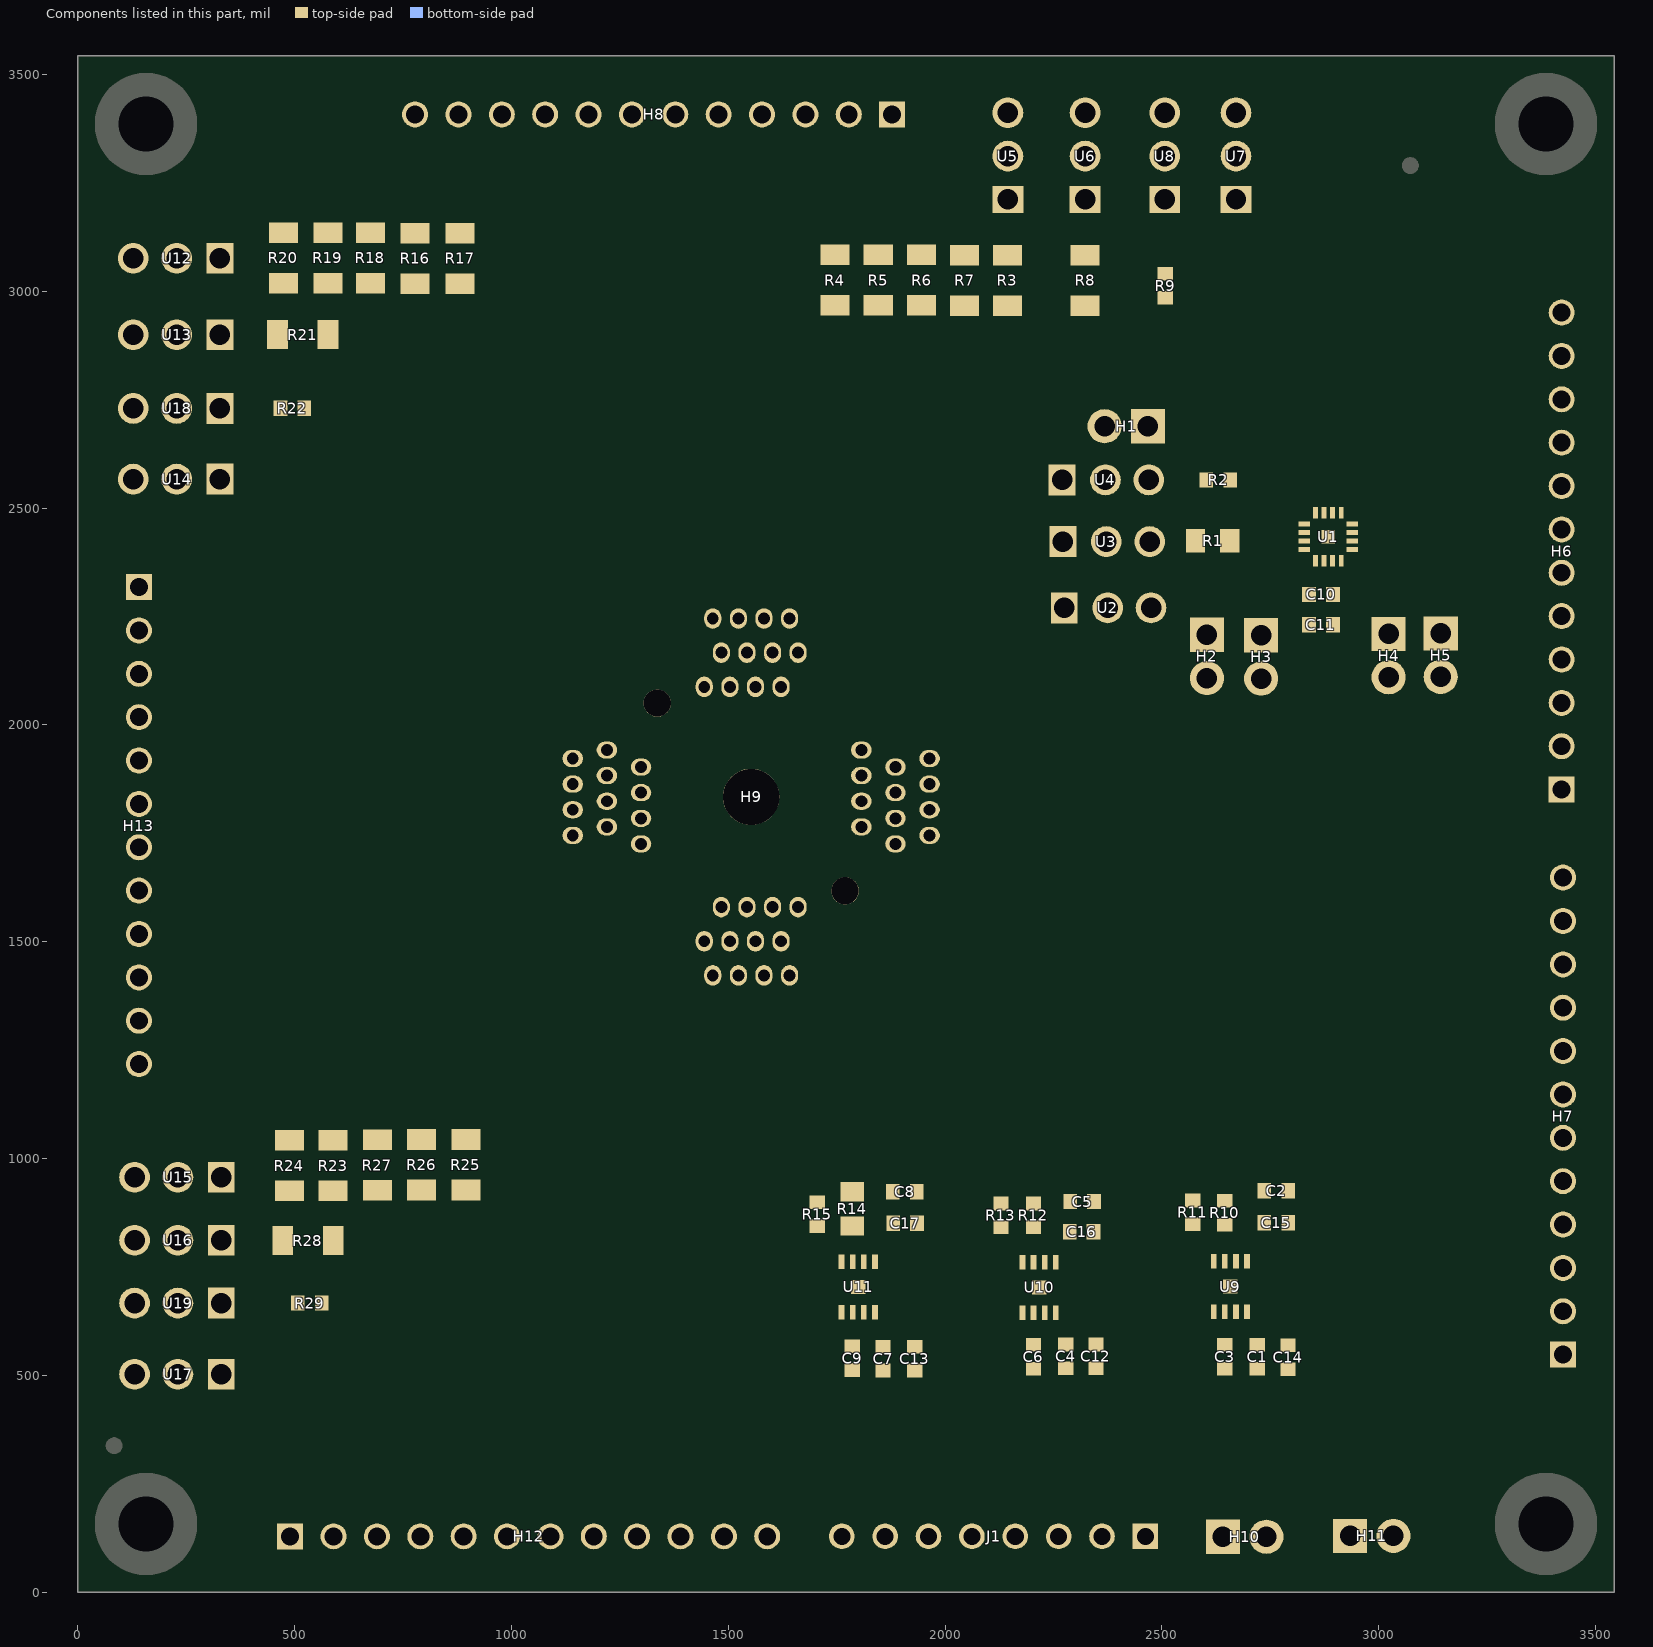
[diagram p0: the components of this part, seen from the top]
# Altium PCB MISC79022.pcbdoc (part 3 of 3)
Units mil, origin at the board's own origin, x right, y up, seen from the top; angles counter-clockwise.
Board outline 3543.31 x 3543.31 mil, 2 copper layers (Top Layer, Bottom Layer); 79 components, 75 nets, 320 pads, 1402 vias.

## Polygon pours and split planes (outlines as drawn)
AVSS on Top Layer "Bottom Layer-No Net" (solid, remove dead copper, pour order 1019): -259,3417.61 -237,3395.61 -237,-231.39 3714,-231.39 3804,-141.39 3860,-85.39 3860,70.61 3860,3854.61 3748,3966.61 3659,4055.61 3614,4055.61 -12,4055.61 -225,3842.61 -270,3797.61 -270,3551.61
3.3V on Top Layer "Bottom Layer-No Net" (solid, remove dead copper, pour order 1018): 2331,152 2331,81 2340,72 2351,61 2394,61 2797,61 2809,73 2818,82 2818,124 2818,276 2912,370 3013,471 3323,471 3444,471 3457,484 3464,491 3464,499 3464,576 3455,585 3437,585 3031,585 2967,649 2952,664 2696,664 2671,664 2668,661 2665,658 2665,652 2665,628 2670,623 2689,604 2689,585 2689,568 2696,561 2700,557 2719,557 2815,557 2833,539 2837,535 2837,521 2837,484 2815,462 2800,447 2686,447 2545,447 2515,477 2497,495 2497,546 2497,612 2468,641 2448,661 2256,661 2232,661 2229,658 2223,652 2223,646 2223,627 2237,613 2243,607 2243,595 2243,575 2255,563 2260,558 2269,558 2367,558 2379,546 2382,543 2382,528 2382,441 2354,413 2342,401 2293,401 2184,401 2143,442 2104,481 2104,545 2104,596 2075,625 2039,661 1841,661 1811,661 1808,658 1806,656 1806,652 1806,622 1818,610 1825,603 1825,594 1825,567 1833,559 1843,549 1852,549 1961,549 1976,534 1999,511 1999,477 1999,373 2020,352 2106,266 2181,266 2269,266 2308,227 2331,204 2331,153
LDO_AVDD on Top Layer "Bottom Layer-No Net" (solid, remove dead copper, pour order 1017): 2624,943 2624,894 2628,890 2634,884 2645,884 2675,884 2683,876 2690,869 2690,851 2690,825 2673,808 2664,799 2664,785 2664,751 2666,749 2668,747 2671,747 2726,747 2734,755 2754,775 2754,837 2754,988 2740,1002 2729,1013 2718,1013 2660,1013 2647,1000 2624,977 2624,944
LDO_DVDDIO on Top Layer "Bottom Layer-No Net" (solid, remove dead copper, pour order 1016): 2222,777 2222,750 2224,748 2227,745 2232,745 2281,745 2289,753 2306,770 2306,824 2306,968 2299,975 2293,981 2282,981 2199,981 2194,976 2183,965 2183,941 2183,894 2190,887 2195,882 2210,882 2225,882 2233,874 2240,867 2240,855 2240,817 2230,807 2222,799 2222,778
LDO_DVDD on Top Layer "Bottom Layer-No Net" (solid, remove dead copper, pour order 1015): 1806,781 1806,754 1808,752 1813,747 1818,747 1862,747 1866,751 1899,784 1899,845 1899,993 1882,1010 1875,1017 1860,1017 1760,1017 1755,1012 1748,1005 1748,975 1748,913 1760,901 1764,897 1779,897 1816,897 1820,893 1828,885 1828,879 1828,821 1821,814 1806,799 1806,784
LDO_DVDDIO on Top Layer "Bottom Layer-No Net" (solid, remove dead copper, pour order 1014): 57,3092 57,2703 71,2689 78,2682 91,2682 255,2682 259,2686 268,2695 268,2756 268,3125 262,3131 255,3138 232,3138 70,3138 62,3130 57,3125 57,3093
DVDDIO on Top Layer "Bottom Layer-No Net" (solid, remove dead copper, pour order 1013): 102,2352 102,2299 113,2288 119,2282 121,2280 487,2280 562,2280 568,2286 588,2306 588,2370 588,2483 618,2513 644,2539 713,2539 789,2539 882,2632 953,2703 953,2931 953,3018 930,3041 926,3045 885,3045 447,3045 442,3040 436,3034 436,3025 436,3005 443,2998 453,2988 470,2988 519,2988 533,2974 545,2962 545,2925 545,2825 526,2806 506,2786 506,2744 506,2669 481,2644 465,2628 406,2628 319,2628 300,2609 295,2604 295,2589 295,2486 280,2471 256,2447 226,2447 147,2447 126,2426 103,2403 103,2357
NetR22_1 on Top Layer "Bottom Layer-No Net" (solid, remove dead copper, pour order 1012): 295,2753 295,2695 299,2691 303,2687 307,2687 471,2687 478,2694 485,2701 485,2715 485,2781 479,2787 475,2791 460,2791 310,2791 302,2783 296,2777 296,2755
NetR21_1 on Top Layer "Bottom Layer-No Net" (solid, remove dead copper, pour order 1011): 297,2918 297,2852 300,2849 311,2838 317,2838 478,2838 481,2841 486,2846 486,2868 486,2944 476,2954 473,2957 440,2957 311,2957 302,2948 296,2942 296,2919
NetR16_1 on Top Layer "Bottom Layer-No Net" (solid, remove dead copper, pour order 1010): 293,3099 293,3041 300,3034 306,3028 328,3028 395,3028 401,3034 405,3038 405,3062 405,3080 425,3100 434,3109 469,3109 913,3109 923,3119 926,3122 926,3193 906,3213 891,3228 844,3228 349,3228 319,3198 293,3172 293,3100
LDO_DVDD on Top Layer "Bottom Layer-No Net" (solid, remove dead copper, pour order 1009): 71,975 71,646 85,632 93,624 111,624 246,624 250,628 264,642 264,671 264,1006 250,1020 243,1027 223,1027 95,1027 86,1018 71,1003 71,975
DVDD on Top Layer "Bottom Layer-No Net" (solid, remove dead copper, pour order 1008): 298,506 298,452 310,440 320,430 348,430 581,430 857,706 945,794 945,917 945,939 936,948 926,958 895,958 460,958 454,952 451,949 451,940 451,905 456,900 463,893 476,893 526,893 543,876 561,858 561,831 561,744 551,734 546,729 546,680 546,609 523,586 511,574 395,574 317,574 305,562 298,555 298,508
NetR29_1 on Top Layer "Bottom Layer-No Net" (solid, remove dead copper, pour order 1007): 299,685 299,623 306,616 315,607 333,607 504,607 516,619 525,628 525,648 525,694 517,702 504,715 475,715 311,715 304,708 299,703 299,686
NetR28_1 on Top Layer "Bottom Layer-No Net" (solid, remove dead copper, pour order 1006): 297,830 297,769 305,761 314,752 325,752 491,752 497,758 500,761 500,778 500,854 495,859 488,866 475,866 309,866 303,860 297,854 297,830
NetR23_1 on Top Layer "Bottom Layer-No Net" (solid, remove dead copper, pour order 1005): 297,983 297,920 299,918 307,910 314,910 398,910 407,919 418,930 418,960 418,993 434,1009 442,1017 531,1017 931,1017 939,1025 943,1029 943,1063 943,1117 931,1129 925,1135 854,1135 337,1135 315,1113 297,1095 297,987
LDO_AVDD on Top Layer "Bottom Layer-No Net" (solid, remove dead copper, pour order 1004): 2078,3431 2078,3299 2095,3282 2102,3275 2137,3275 2559,3275 2567,3283 2578,3294 2578,3327 2578,3458 2567,3469 2557,3479 2533,3479 2098,3479 2088,3469 2078,3459 2078,3432
NetR9_1 on Top Layer "Bottom Layer-No Net" (solid, remove dead copper, pour order 1003): 2463,3213 2463,3043 2471,3035 2482,3024 2495,3024 2531,3024 2543,3036 2565,3058 2565,3082 2565,3230 2558,3237 2551,3244 2529,3244 2475,3244 2466,3235 2463,3232 2463,3213
NetR8_1 on Top Layer "Bottom Layer-No Net" (solid, remove dead copper, pour order 1002): 2259,3212 2259,3077 2266,3070 2278,3058 2299,3058 2379,3058 2386,3065 2392,3071 2392,3119 2392,3222 2375,3239 2371,3243 2348,3243 2276,3243 2265,3232 2259,3226 2259,3214
AVDD on Top Layer "Bottom Layer-No Net" (solid, remove dead copper, pour order 1001): 1706,2968 1706,2908 1716,2898 1736,2878 1775,2878 2665,2878 2688,2901 2730,2943 2730,3138 2730,3225 2714,3241 2709,3246 2691,3246 2628,3246 2621,3239 2616,3234 2616,3221 2616,3059 2578,3021 2551,2994 2260,2994 1716,2994 1710,2988 1706,2984 1706,2968
NetR3_1 on Top Layer "Bottom Layer-No Net" (solid, remove dead copper, pour order 1000): 1710,3118 1710,3097 1710,3063 1713,3060 1715,3058 1717,3058 2178,3058 2182,3062 2189,3069 2189,3082 2189,3240 2185,3244 2180,3249 2162,3249 2088,3249 2080,3241 2073,3234 2073,3227 2073,3188 2065,3180 2042,3157 1964,3157 1727,3157 1717,3147 1710,3140 1710,3120
AVSS on Bottom Layer "Bottom Layer-No Net" (solid, remove dead copper, pour order 1023): -341,3525 -341,-24 -106,-259 -17,-348 196,-348 3868,-348 4013,-203 4125,-91 4125,178 4125,3223 3722,3626 3588,3760 2715,3760 -116,3760 -318,3558
LDO_AVDD on Bottom Layer "Bottom Layer-No Net" (solid, remove dead copper, pour order 1022): 2638,1000 2638,962 2649,951 2662,938 2690,938 2743,938 2752,947 2760,955 2760,960 2760,1001 2739,1022 2735,1026 2724,1026 2664,1026 2638,1000
LDO_DVDDIO on Bottom Layer "Bottom Layer-No Net" (solid, remove dead copper, pour order 1021): 2192,976 2192,933 2195,930 2205,920 2214,920 2287,920 2293,926 2296,929 2296,933 2296,978 2286,988 2277,997 2263,997 2207,997 2199,989 2192,982 2192,977
LDO_DVDD on Bottom Layer "Bottom Layer-No Net" (solid, remove dead copper, pour order 1020): 1761,1011 1761,965 1766,960 1771,955 1777,955 1875,955 1880,960 1886,966 1886,971 1886,1005 1877,1014 1871,1020 1849,1020 1766,1020 1762,1016 1761,1015 1761,1012

## Keep-outs
Keep-Out Layer:
  the board outline again, w10

## Silkscreen, mask and mechanical layers (free items; w line width, h text height)
Top Overlay:
  text "NEG1" at 994,3231 h45 r90
  text "NEG0" at 1094,3228 h45 r90
  text "AVSS" at 791,3227 h45 r90
  text "NEG2" at 894,3227 h45 r90
  text "NEG3" at 1293,3226 h45 r90
  text "NEG5" at 1196,3225 h45 r90
  text "NEG4" at 1396,3224 h45 r90
  text "NEG6" at 1492,3222 h45 r90
  text "NEG7" at 1598,3221 h45 r90
  text "NEG8" at 1793,3221 h45 r90
  text "NEG9" at 1694,3220 h45 r90
  text "AVSS" at 1895,3216 h45 r90
  text "DAC_REF_OUT" at 3045,2940 h45
  text "DAC_DATA_OUT" at 3013,2849 h45
  text "DAC_IN" at 3194,2749 h45
  text "DAC_CLK" at 3151,2646 h45
  text "DAC_EN" at 3175,2549 h45
  text "DAC_OUT7" at 3123,2440 h45
  text "DAC_OUT6" at 3126,2347 h45
  text "DVDDIO" at 224,2311 h45
  text "3V3" at 3273,2238 h45
  text "DSIGN" at 236,2210 h45
  text "AVDD" at 3247,2144 h45
  text "RST" at 240,2107 h45
  text "DAC_ADC_IN" at 3104,2018 h45
  text "3V3" at 241,2009 h45
  text "AVSS" at 3233,1935 h45
  text "3V3" at 244,1910 h45
  text "AVSS" at 3239,1837 h45
  text "AVSS" at 244,1808 h45
  text "AVSS" at 246,1708 h45
  text "OTA_BIAS" at 3143,1640 h45
  text "DVDD" at 247,1605 h45
  text "VCLAMP" at 3177,1534 h45
  text "DVDD" at 249,1503 h45
  text "VBIASP" at 3196,1432 h45
  text "AVSS" at 253,1407 h45
  text "VBIASN" at 3192,1330 h45
  text "S1" at 264,1308 h45
  text "ADC_IN" at 3195,1244 h45
  text "S2" at 263,1204 h45
  text "AVSS" at 3226,1130 h45
  text "SAMPLE" at 3175,1035 h45
  text "HEAD" at 3231,928 h45
  text "AVDD" at 3227,840 h45
  text "AVDD" at 3229,728 h45
  text "AVSS" at 3231,628 h45
  text "3V3" at 3273,535 h45
  text "POS1" at 1500,214 h45 r90
  text "POS0" at 1409,211 h45 r90
  text "POS2" at 1305,210 h45 r90
  text "S0" at 605,209 h45 r90
  text "POS5" at 906,209 h45 r90
  text "AVSS" at 1596,209 h45 r90
  text "POS9" at 806,208 h45 r90
  text "POS3" at 1210,208 h45 r90
  text "LDO_AVDD" at 2067,208 h45 r90
  text "AVSS" at 2179,208 h45 r90
  text "3V3" at 2650,208 h45
  text "POS7" at 703,207 h45 r90
  text "POS6" at 1004,207 h45 r90
  text "POS4" at 1100,207 h45 r90
  text "GND" at 2951,206 h45
  text "LDO_DVDDIO" at 1974,205 h45 r90
  text "3V3" at 2381,205 h45 r90
  text "POS8" at 500,204 h45 r90
  text "AVSS" at 2274,204 h45 r90
  text "3V3" at 2477,204 h45 r90
  text "EN_LDO" at 1767,202 h45 r90
  text "LDO_DVDD" at 1869,202 h45 r90